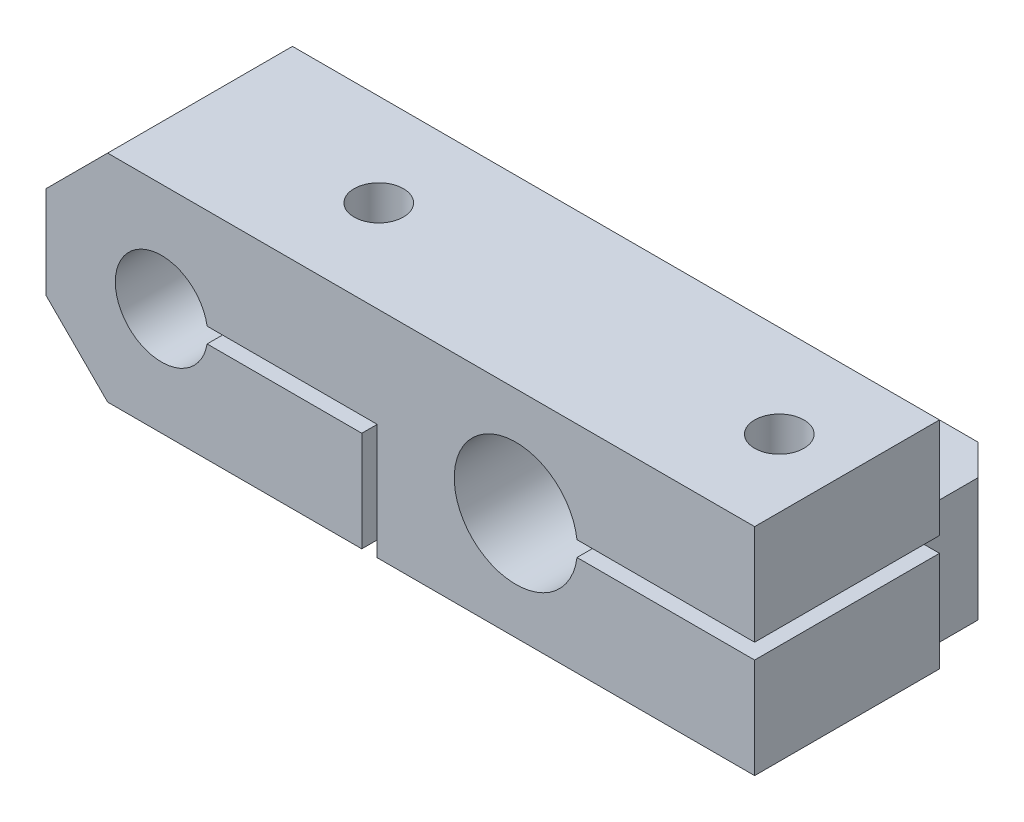
SolidWorks part; units mm, degrees
material "6061 合金"
ref_plane "Front Plane" through (0, 0, 0) normal (0, 0, 1) x (1, 0, 0)
ref_plane "Top Plane" through (0, 0, 0) normal (0, 1, 0) x (1, 0, 0)
ref_plane "Right Plane" through (0, 0, 0) normal (1, 0, 0) x (0, 0, -1)
sketch "Sketch1" plane through (0, 0, 0) normal (0, 0, 1) x (1, 0, 0)
  line L0 (0, 0) -> (50000, 0) construction
  line L1 (-14.5, 7.5) -> (14.5, 7.5)
  line L2 (-14.5, 7.5) -> (-14.5, -7.5)
  line L3 (-14.5, -7.5) -> (14.5, -7.5)
  line L4 (14.5, 7.5) -> (14.5, -7.5)
  line L5 (-14.5, 7.5) -> (14.5, -7.5) construction
  line L6 (-14.5, -7.5) -> (14.5, 7.5) construction
  line L7 (0, 0) -> (0, -50000) construction
  circle A1 centre (6.75, 0) radius 2
  circle A2 centre (-4.75, 0) radius 1.5
  point P0 (0, 0)
  point P10 (0, -7.5)
  dimension "D1" = 4
  dimension "D2" = 4.75
  dimension "D5" = 6.75
  dimension "D3" = 29
  dimension "D4" = 15
extrude "Boss-Extrude1" add sketch "Sketch1" along normal blind 13
sketch "Sketch3" plane through (0, -7.5, 0) normal (0, -1, 0) x (1, 0, 0)
  line L0 (14.5, 0) -> (-14.5, 0) construction
  line L1 (14.5, 13) -> (9.75, 13)
  line L2 (14.5, 13) -> (14.5, 0)
  line L3 (14.5, 0) -> (9.75, 0)
  line L4 (9.75, 13) -> (9.75, 0)
  line L6 (-14.5, 13) -> (3.75, 13)
  line L7 (-14.5, 13) -> (-14.5, 0)
  line L8 (-14.5, 0) -> (3.75, 0)
  line L9 (3.75, 13) -> (3.75, 0)
  dimension "D1" = 6
  dimension "D2" = 4.75
extrude "Cut-Extrude1" cut sketch "Sketch3" against normal blind 4
sketch "Sketch5" plane through (0, 0, 0) normal (0, 0, -1) x (-1, 0, 0)
  line L0 (14.5, 7.5) -> (14.5, -3.5) construction
  line L1 (-14.5, 7.5) -> (14.5, 7.5)
  line L2 (-14.5, 7.5) -> (-14.5, 3.5)
  line L3 (-14.5, 3.5) -> (14.5, 3.5)
  line L4 (14.5, 7.5) -> (14.5, 3.5)
  line L5 (14.5, -3.5) -> (-3.75, -3.5) construction
  dimension "D1" = 7
extrude "Cut-Extrude2" cut sketch "Sketch5" against normal blind 27
sketch "Sketch6" plane through (0, 0, 0) normal (0, 0, -1) x (-1, 0, 0)
  line L5 (0, 0) -> (0, 50000) construction
  line L6 (14.5, 3.5) -> (14.5, -3.5)
  line L7 (14.5, -3.5) -> (13, -3.5)
  line L8 (13, 3.5) -> (13, -3.5)
  line L9 (14.5, 3.5) -> (13, 3.5)
extrude "Cut-Extrude3" cut sketch "Sketch6" against normal blind 27
sketch "Sketch7" plane through (0, 0, 0) normal (0, 0, -1) x (-1, 0, 0)
  line L0 (-14.5, -3.5) -> (-14.5, 3.5) construction
  line L1 (-14.5, 3.5) -> (13, 3.5)
  line L2 (-14.5, -3.5) -> (-14.5, 3.5)
  line L3 (-14.5, -3.5) -> (13, -3.5)
  line L4 (13, 3.5) -> (13, -3.5)
extrude "Cut-Extrude4" cut sketch "Sketch7" against normal blind 7
chamfer "Chamfer1" distance 6 distance2 4 1 edges at (6.75, -7.5, 13)
sketch "Sketch8" plane through (0, 0, 7) normal (0, 0, -1) x (-1, 0, 0)
  line L0 (0, 0) -> (-50000, 0) construction
  line L1 (-1.75, -3.5) -> (-1.75, -0.25)
  line L2 (-8, -0.25) -> (-14.5, -0.25)
  line L3 (-8, -0.25) -> (-8, 0.25)
  line L4 (-8, 0.25) -> (-14.5, 0.25)
  line L5 (-14.5, -3.5) -> (-14.5, 3.5) construction
  line L8 (357.6967, 900.1167) -> (-2.5387, -0.4719) construction
  line L9 (3.75, 0.25) -> (-2.25, 0.25)
  line L10 (-14.5, -0.25) -> (-14.5, 0.25)
  line L11 (-3.75, -3.5) -> (-17957.3079, -44887.3946) construction
  line L12 (3.75, 0.25) -> (3.75, -0.25)
  line L15 (-3.75, -3.5) -> (13, -3.5) construction
  line L16 (-1.75, -0.25) -> (3.75, -0.25)
  line L21 (-2.25, 0.25) -> (-2.25, -3.5)
  line L22 (-2.25, -3.5) -> (-1.75, -3.5)
  circle A1 centre (4.75, 0) radius 1.5 construction
  point P3 (-10.5, 0)
  point P10 (2.4343, 0)
  dimension "D6" = 7
  dimension "D1" = 0.5
  dimension "D3" = 0.5
  dimension "D4" = 6
  dimension "D5" = 0.5
extrude "Cut-Extrude5" cut sketch "Sketch8" against normal blind 9
sketch "Sketch9" plane through (0, -3.5, 0) normal (0, -1, 0) x (1, 0, 0)
  line L0 (-12.5, 10) -> (49987.5, 10) construction
  line L1 (-13, 13) -> (-13, 7) construction
  line L3 (14.5, 7) -> (14.5, 13) construction
  circle A0 centre (12.3, 10) radius 1.25
  circle A1 centre (-0.7, 10) radius 1.25
  point P4 (-13, 10)
  dimension "D1" = 2.5
  dimension "D2" = 13
  dimension "D3" = 2.2
extrude "Cut-Extrude6" cut sketch "Sketch9" against normal up to surface (3.25 mm away) up to face at (-0.7605, -0.25, 10)
sketch "Sketch12" plane through (0, 0, 13) normal (0, 0, 1) x (1, 0, 0)
  line L0 (1.75, -3.5) -> (-13, -3.5) construction
  line L1 (-13, 3.5) -> (-10, 3.5)
  line L2 (-13, 3.5) -> (-13, -3.5)
  line L3 (-13, -3.5) -> (-10, -3.5)
  line L4 (-10, 3.5) -> (-10, -3.5)
  dimension "D1" = 3
extrude "Cut-Extrude8" cut sketch "Sketch12" against normal blind 8
sketch "Sketch13" plane through (0, -7.5, 0) normal (0, -1, 0) x (1, 0, 0)
  line L0 (6.75, 0) -> (6.75, 50000) construction
  line L1 (3.75, 0) -> (9.75, 0) construction
  line L2 (14.5, 13) -> (9.75, 13) construction
  circle A0 centre (6.75, 3) radius 1.5
  point P4 (6.75, 0)
  dimension "D1" = 3
  dimension "D2" = 10
extrude "Cut-Extrude9" cut sketch "Sketch13" against normal blind 8
chamfer "Chamfer3" distance 1 angle 45 2 edges at (9.75, -5.5, 0) (3.75, -5.5, 0)
sketch "Sketch17" plane through (0, 0, 7) normal (0, 0, -1) x (-1, 0, 0)
  line L0 (-1.75, -3.5) -> (10, -3.5) construction
  line L1 (10, 3.5) -> (8.5, 3.5)
  line L2 (10, 3.5) -> (10, -3.5)
  line L3 (10, -3.5) -> (8.5, -3.5)
  line L4 (8.5, 3.5) -> (8.5, -3.5)
  dimension "D1" = 1.5
extrude "Cut-Extrude11" cut sketch "Sketch17" against normal blind 9
chamfer "Chamfer4" distance 2 angle 45 2 edges at (-8.5, 3.5, 10) (-8.5, -3.5, 10)
hole_wizard "M2 Tapped Hole1" positions "Sketch19" profile "Sketch18" tap size "M2" standard "Gb" end condition through all
sketch "Sketch19" plane through (0, 3.5, 0) normal (0, 1, 0) x (1, 0, 0)
  point P0 (-0.7, -10)
  point P3 (12.3, -10)
sketch "Sketch18" plane through (-0.7, 3.5, 10) normal (1, 0, 0) x (0, 0, 1)
  line L0 (0, 0) -> (0, 11)
  line L1 (0, 11) -> (0.8, 11)
  line L2 (0.8, 11) -> (0.8, 0)
  line L5 (0.8, 0) -> (0, 0)
  line L11 (0, -6.35) -> (0, 107.95) construction
  dimension "通孔螺纹孔钻头直径" = 1.6
  dimension "通孔螺纹孔钻头深度" = 11
cosmetic thread "Cosmetic Thread1" parameters "D2"=2
cosmetic thread "Cosmetic Thread2" parameters "D2"=2
